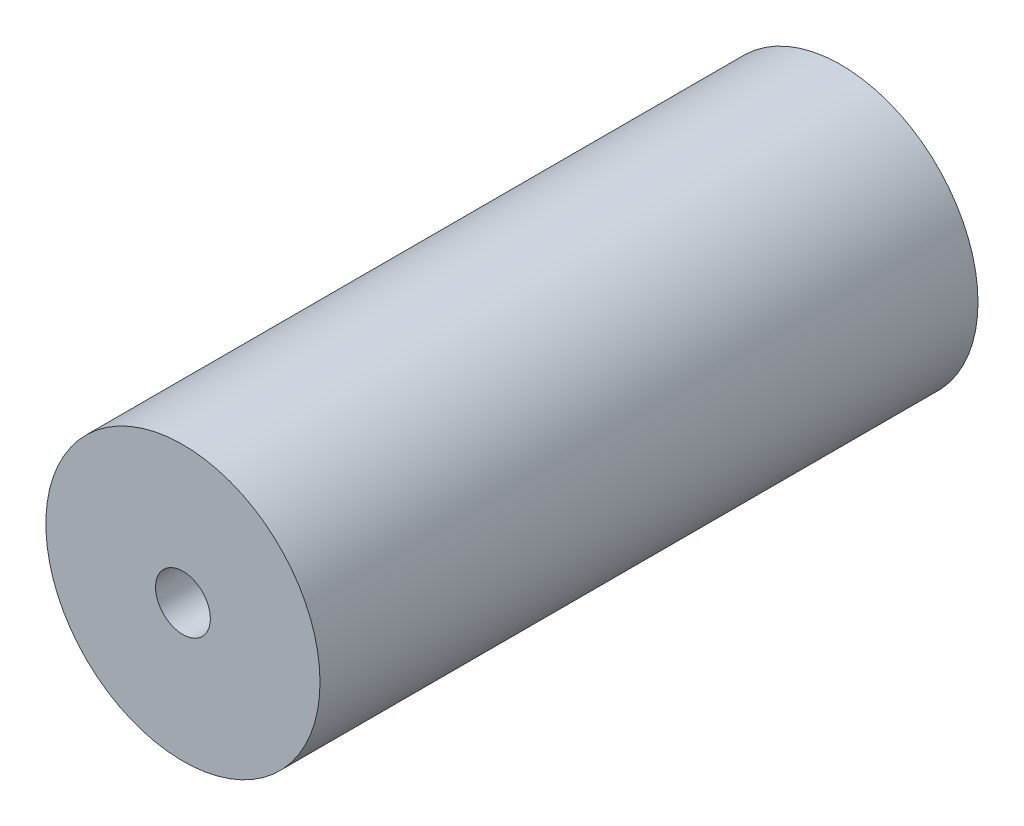
SolidWorks part; units mm, degrees
material "6061 Alloy"
ref_plane "Front Plane" through (0, 0, 0) normal (0, 0, 1) x (1, 0, 0)
ref_plane "Top Plane" through (0, 0, 0) normal (0, 1, 0) x (1, 0, 0)
ref_plane "Right Plane" through (0, 0, 0) normal (1, 0, 0) x (0, 0, -1)
sketch "Sketch 1" plane through (0, 0, 0) normal (0, 0, 1) x (1, 0, 0)
  circle A0 centre (0, 0) radius 12.5
  dimension "D1" = 25
extrude "Boss-Extrude 1" add sketch "Sketch 1" along normal blind 60
hole_wizard "M6 Tapped Hole 1" positions "Sketch 3" profile "Sketch 2" tap size "M6" standard "GB"
sketch "Sketch 3" plane through (0, 0, 60) normal (0, 0, 1) x (1, 0, 0)
  point P1 (0, 0)
sketch "Sketch 2" plane through (0, 0, 60) normal (1, 0, 0) x (0, -1, 0)
  line L0 (0, 0) -> (0, 16.5022)
  line L1 (0, 16.5022) -> (2.5, 15)
  line L2 (2.5, 15) -> (2.5, 0)
  line L5 (2.5, 0) -> (0, 0)
  line L10 (0, 16.5022) -> (-2.5, 15) construction
  line L11 (0, -6.35) -> (0, 107.95) construction
  dimension "螺孔鑽直徑" = 5
  dimension "螺孔鑽深度" = 15
  dimension "導頭角度" = 118
cosmetic thread "Cosmetic Thread 1" parameters "D1"=12, "D2"=6
hole_wizard "M6 Tapped Hole 2" positions "Sketch 5" profile "Sketch 4" tap size "M6" standard "GB"
sketch "Sketch 5" plane through (0, 0, 0) normal (0, 0, -1) x (-1, 0, 0)
  point P2 (0, 0)
sketch "Sketch 4" plane through (0, 0, 0) normal (1, 0, 0) x (0, 1, 0)
  line L0 (0, 0) -> (0, 16.5022)
  line L1 (0, 16.5022) -> (2.5, 15)
  line L2 (2.5, 15) -> (2.5, 0)
  line L5 (2.5, 0) -> (0, 0)
  line L10 (0, 16.5022) -> (-2.5, 15) construction
  line L11 (0, -6.35) -> (0, 107.95) construction
  dimension "螺孔鑽直徑" = 5
  dimension "螺孔鑽深度" = 15
  dimension "導頭角度" = 118
cosmetic thread "Cosmetic Thread 2" parameters "D1"=12, "D2"=6
